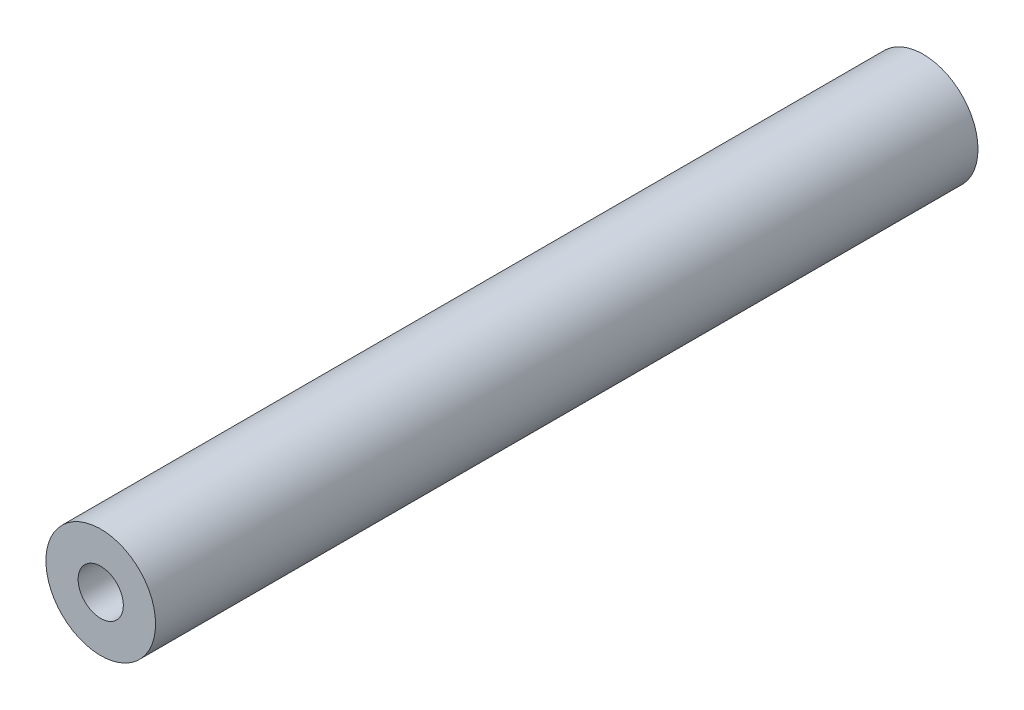
SolidWorks part; units mm, degrees
ref_plane "前视基准面" through (0, 0, 0) normal (0, 0, 1) x (1, 0, 0)
ref_plane "上视基准面" through (0, 0, 0) normal (0, 1, 0) x (1, 0, 0)
ref_plane "右视基准面" through (0, 0, 0) normal (1, 0, 0) x (0, 0, -1)
other "Configuration Table"
sketch "草图1" plane through (0, 0, 0) normal (0, 0, 1) x (1, 0, 0)
  circle A0 centre (0, 0) radius 4
  circle A1 centre (0, 0) radius 1.65
  point P0 (0, 0)
  dimension "D1" = 3.3
  dimension "D2" = 8
extrude "凸台-拉伸1" add sketch "草图1" against normal mid plane 60
